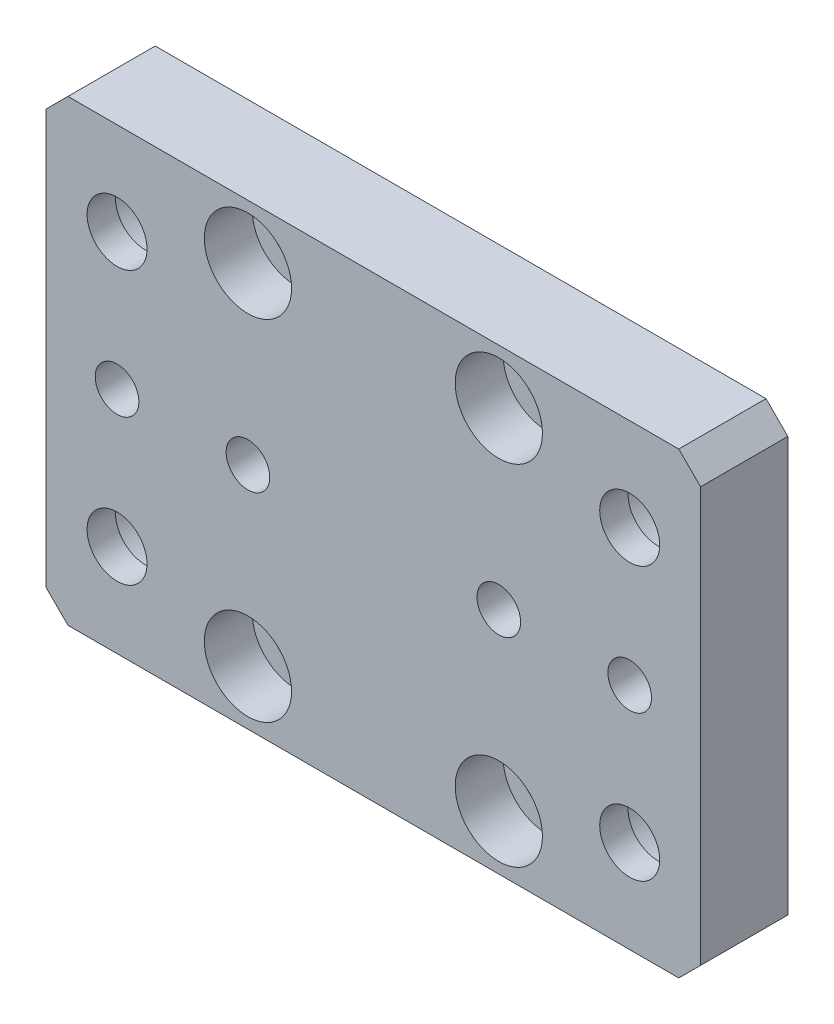
SolidWorks part; units mm, degrees
material "AL6061"
ref_plane "Front" through (0, 0, 0) normal (0, 0, 1) x (1, 0, 0)
ref_plane "Top" through (0, 0, 0) normal (0, 1, 0) x (1, 0, 0)
ref_plane "Right" through (0, 0, 0) normal (1, 0, 0) x (0, 0, -1)
sketch "Sketch1" plane through (0, 0, 0) normal (0, 0, 1) x (1, 0, 0)
  line L1 (0, 0) -> (60, 0)
  line L2 (0, 0) -> (0, 42)
  line L3 (0, 42) -> (60, 42)
  line L4 (60, 0) -> (60, 42)
  dimension "D1" = 42
  dimension "D2" = 60
extrude "Boss-Extrude1" add sketch "Sketch1" along normal blind 8
hole_wizard "CBORE for M4 Hex Socket Head Cap Screw2" positions "Sketch2" profile "Sketch3" counterbore size "M4" standard "ISO" end condition through all
sketch "Sketch2" plane through (0, 0, 8) normal (0, 0, 1) x (1, 0, 0)
  line L0 (30, 42) -> (30, 0) construction
  line L1 (60, 42) -> (0, 42) construction
  line L2 (0, 0) -> (60, 0) construction
  line L5 (0, 21) -> (60, 21) construction
  line L6 (0, 42) -> (0, 0) construction
  line L7 (60, 0) -> (60, 42) construction
  point P18 (18.5, 37)
  point P21 (18.5, 5)
  point P22 (41.5, 5)
  point P23 (41.5, 37)
  dimension "D1" = 23
  dimension "D2" = 32
sketch "Sketch3" plane through (41.5, 37, 8) normal (1, 0, 0) x (0, -1, 0)
  line L0 (0, 0) -> (0, 8)
  line L1 (0, 8) -> (2.25, 8)
  line L3 (2.25, 8) -> (2.25, 4.4)
  line L4 (2.25, 4.4) -> (4, 4.4)
  line L5 (4, 4.4) -> (4, 0)
  line L7 (4, 0) -> (0, 0)
  line L11 (0, -6.35) -> (0, 107.95) construction
  dimension "通孔孔直径" = 4.5
  dimension "通孔孔深度" = 8
  dimension "柱形沉头孔直径" = 8
  dimension "柱形沉头孔深度" = 4.4
sketch "Sketch4" plane through (0, 0, 8) normal (0, 0, 1) x (1, 0, 0)
  line L0 (18.5, 37) -> (18.5, 5) construction
  line L1 (41.5, 37) -> (41.5, 5) construction
  line L2 (18.5, 21) -> (41.5, 21) construction
  circle A0 centre (18.5, 21) radius 2
  circle A1 centre (41.5, 21) radius 2
  dimension "D1" = 4
extrude "Cut-Extrude1" cut sketch "Sketch4" against normal through all
hole_wizard "CBORE for M5 Hex Socket Head Cap Screw1" positions "Sketch5" profile "Sketch6" counterbore size "M5" standard "ISO" end condition through all
sketch "Sketch5" plane through (0, 0, 0) normal (0, 0, 1) x (1, 0, 0)
  line L0 (30, 42) -> (30, 0) construction
  line L1 (60, 42) -> (0, 42) construction
  line L2 (0, 0) -> (60, 0) construction
  line L5 (0, 21) -> (60, 21) construction
  line L6 (0, 42) -> (0, 0) construction
  line L7 (60, 0) -> (60, 42) construction
  line L10 (6.5, 42) -> (6.5, 0) construction
  line L11 (53.5, 42) -> (53.5, 0) construction
  point P26 (6.5, 33.5)
  point P29 (6.5, 8.5)
  point P32 (53.5, 8.5)
  point P33 (53.5, 33.5)
  dimension "D1" = 6.5
  dimension "D2" = 25
sketch "Sketch6" plane through (53.5, 33.5, 0) normal (1, 0, 0) x (0, 1, 0)
  line L0 (0, 0) -> (0, 8)
  line L1 (0, 8) -> (2.75, 8)
  line L3 (2.75, 8) -> (2.75, 5.4)
  line L4 (2.75, 5.4) -> (5, 5.4)
  line L5 (5, 5.4) -> (5, 0)
  line L7 (5, 0) -> (0, 0)
  line L11 (0, -6.35) -> (0, 107.95) construction
  dimension "通孔孔直径" = 5.5
  dimension "通孔孔深度" = 8
  dimension "柱形沉头孔直径" = 10
  dimension "柱形沉头孔深度" = 5.4
sketch "Sketch7" plane through (0, 0, 8) normal (0, 0, 1) x (1, 0, 0)
  line L0 (30, 42) -> (30, 0) construction
  line L1 (60, 42) -> (0, 42) construction
  line L2 (0, 0) -> (60, 0) construction
  line L3 (0, 21) -> (60, 21) construction
  line L4 (0, 42) -> (0, 0) construction
  line L5 (60, 0) -> (60, 42) construction
  line L6 (6.5, 33.5) -> (6.5, 8.5) construction
  circle A0 centre (6.5, 21) radius 2
  circle A1 centre (53.5, 21) radius 2
  dimension "D1" = 4
extrude "Cut-Extrude2" cut sketch "Sketch7" against normal through all
chamfer "Chamfer1" distance 2 angle 45 4 edges at (60, 42, 4) (60, 0, 4) (0, 42, 4) (0, 0, 4)
